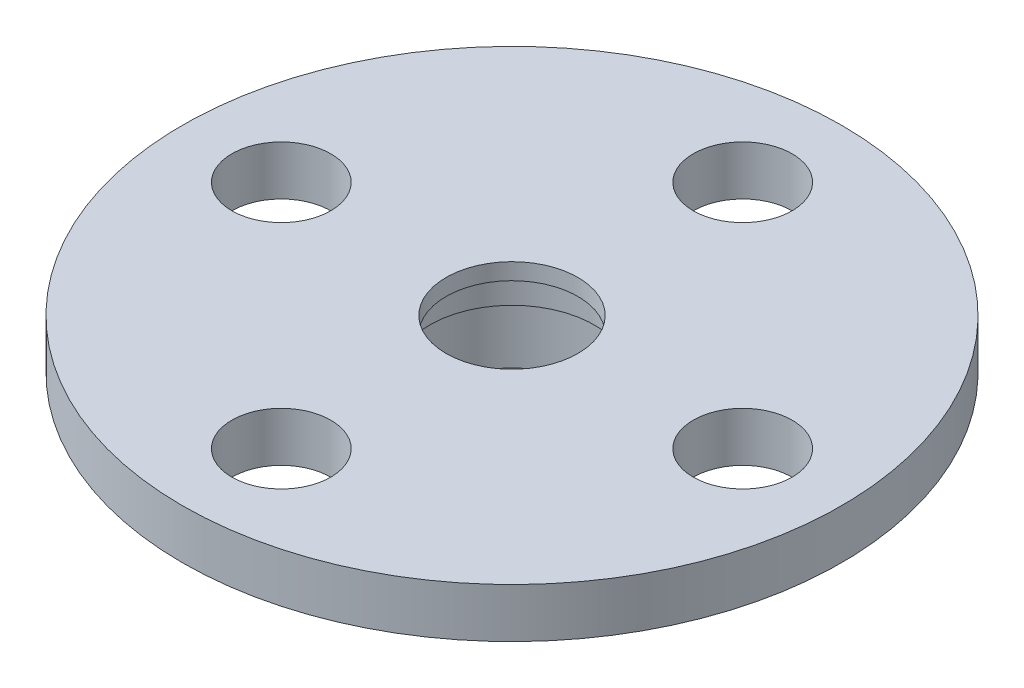
SolidWorks part; units mm, degrees
material "SUS304"
ref_plane "Front Plane" through (0, 0, 0) normal (0, 0, 1) x (1, 0, 0)
ref_plane "Top Plane" through (0, 0, 0) normal (0, 1, 0) x (1, 0, 0)
ref_plane "Right Plane" through (0, 0, 0) normal (1, 0, 0) x (0, 0, -1)
other "Configuration Table"
sketch "Sketch1" plane through (0, 0, 0) normal (0, 0, 1) x (1, 0, 0)
  line L0 (-0.1385, 1.2804) -> (7.8615, 1.2804)
  line L1 (7.8615, 1.2804) -> (7.8615, -0.2196)
  line L2 (7.8615, -0.2196) -> (1.8615, -0.2196)
  line L5 (1.8615, -1.0196) -> (1.8615, -2.2196)
  line L6 (1.8615, -2.2196) -> (0.8615, -2.2196)
  line L7 (0.8615, -2.2196) -> (0.8615, -0.2196)
  line L8 (0.8615, -0.2196) -> (0.3615, -0.2196)
  line L9 (0.3615, -0.2196) -> (0.3615, 0.7804)
  line L10 (0.3615, 0.7804) -> (-0.1385, 0.7804)
  line L11 (-0.1385, 0.7804) -> (-0.1385, 1.2804)
  line L12 (-2.1385, 1.5405) -> (-2.1385, -1.5) construction
  line L13 (1.8615, -1.0196) -> (1.8615, -0.2196)
  point P14 (-0.1385, 1.0304)
  dimension "D1" = 1
  dimension "D2" = 4
  dimension "D3" = 10
  dimension "D4" = 2
  dimension "D5" = 1.5
  dimension "D6" = 2
  dimension "D7" = 0.5
  dimension "D8" = 0
  dimension "D9" = 2.5
revolve "Revolve1" add sketch "Sketch1" angle 360 about L12
sketch "Sketch2" plane through (0, 1.2804, 0) normal (0, 1, 0) x (1, 0, 0)
  circle A1 centre (-2.1385, 0) radius 10 construction
  circle A2 centre (-2.1385, 7) radius 1.5
  circle A8 centre (4.8615, 0) radius 1.5
  circle A9 centre (-2.1385, -7) radius 1.5
  circle A10 centre (-9.1385, 0) radius 1.5
  point P13 (-2.1385, 0)
  point P22 (-2.1385, 0)
  dimension "D1" = 3
  dimension "D3" = 7
  dimension "D2" = 4
extrude "Cut-Extrude1" cut sketch "Sketch2" against normal blind 10
